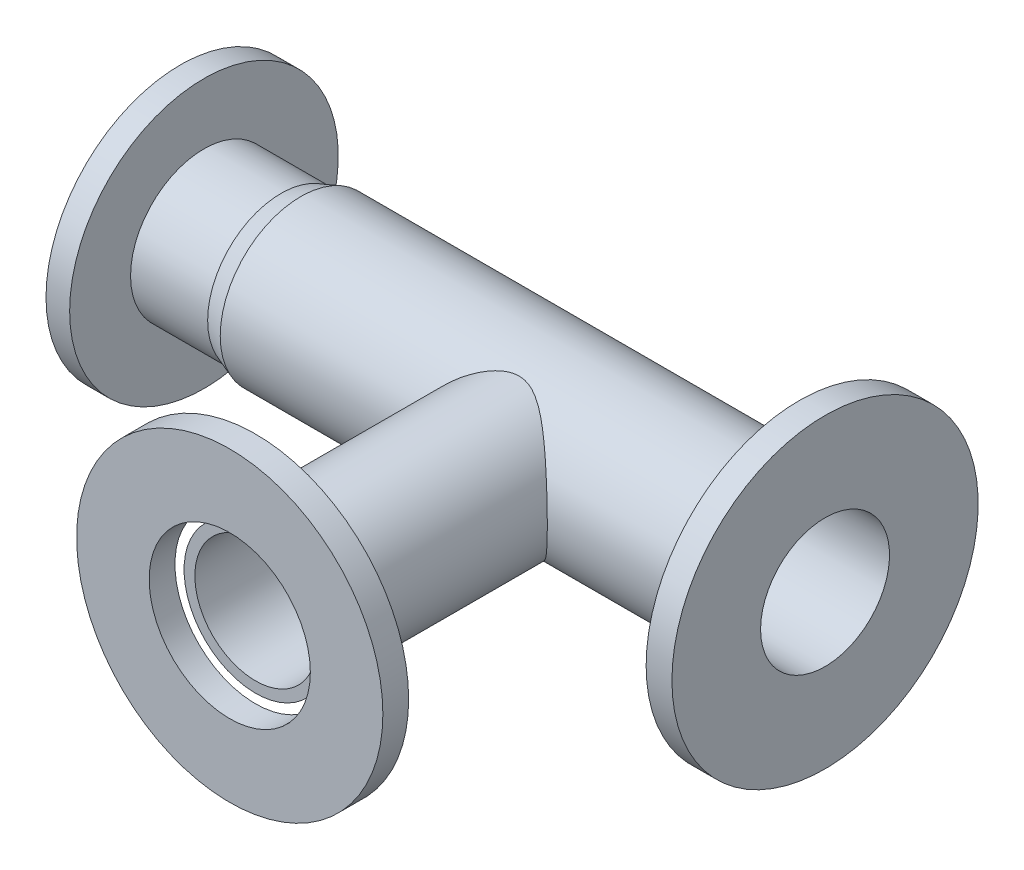
SolidWorks part; units mm, degrees
material "普通碳钢"
ref_plane "Front Plane" through (0, 0, 0) normal (0, 0, 1) x (1, 0, 0)
ref_plane "Top Plane" through (0, 0, 0) normal (0, 1, 0) x (1, 0, 0)
ref_plane "Right Plane" through (0, 0, 0) normal (1, 0, 0) x (0, 0, -1)
sketch "Sketch1" plane through (0, 0, 0) normal (0, 0, 1) x (1, 0, 0)
  line L0 (0, 60) -> (0, 125)
  line L1 (0, 125) -> (22, 125)
  line L2 (22, 125) -> (22, 68.3)
  line L8 (576, 75) -> (576, 142.5)
  line L9 (576, 142.5) -> (600, 142.5)
  line L10 (600, 142.5) -> (600, 60)
  line L11 (600, 60) -> (0, 60)
  line L12 (0, 0) -> (45.6274, 0) construction
  line L13 (576, 75) -> (112.1459, 75)
  line L14 (112.1459, 75) -> (93.7379, 68.3)
  line L15 (93.7379, 68.3) -> (22, 68.3)
  dimension "D1" = 125
  dimension "D2" = 142.5
  dimension "D3" = 22
  dimension "D4" = 24
  dimension "D5" = 60
  dimension "D6" = 20
  dimension "D7" = 75
  dimension "D11" = 600
revolve "Revolve1" add sketch "Sketch1" angle 360 about L12
sketch "Sketch2" plane through (0, 0, 0) normal (0, 0, 1) x (1, 0, 0)
  line L0 (600, -142.5) -> (600, 142.5) construction
  circle A0 centre (350, 0) radius 66.5
  circle A1 centre (350, 0) radius 56.5
  dimension "D1" = 133
  dimension "D2" = 10
  dimension "D3" = 250
extrude "Boss-Extrude1" add sketch "Sketch2" along normal blind 280
sketch "Sketch3" plane through (0, 0, 280) normal (0, 0, 1) x (1, 0, 0)
  circle A0 centre (350, 0) radius 75
  circle A1 centre (350, 0) radius 142.5
  dimension "D1" = 285
extrude "Boss-Extrude2" add sketch "Sketch3" along normal blind 24
